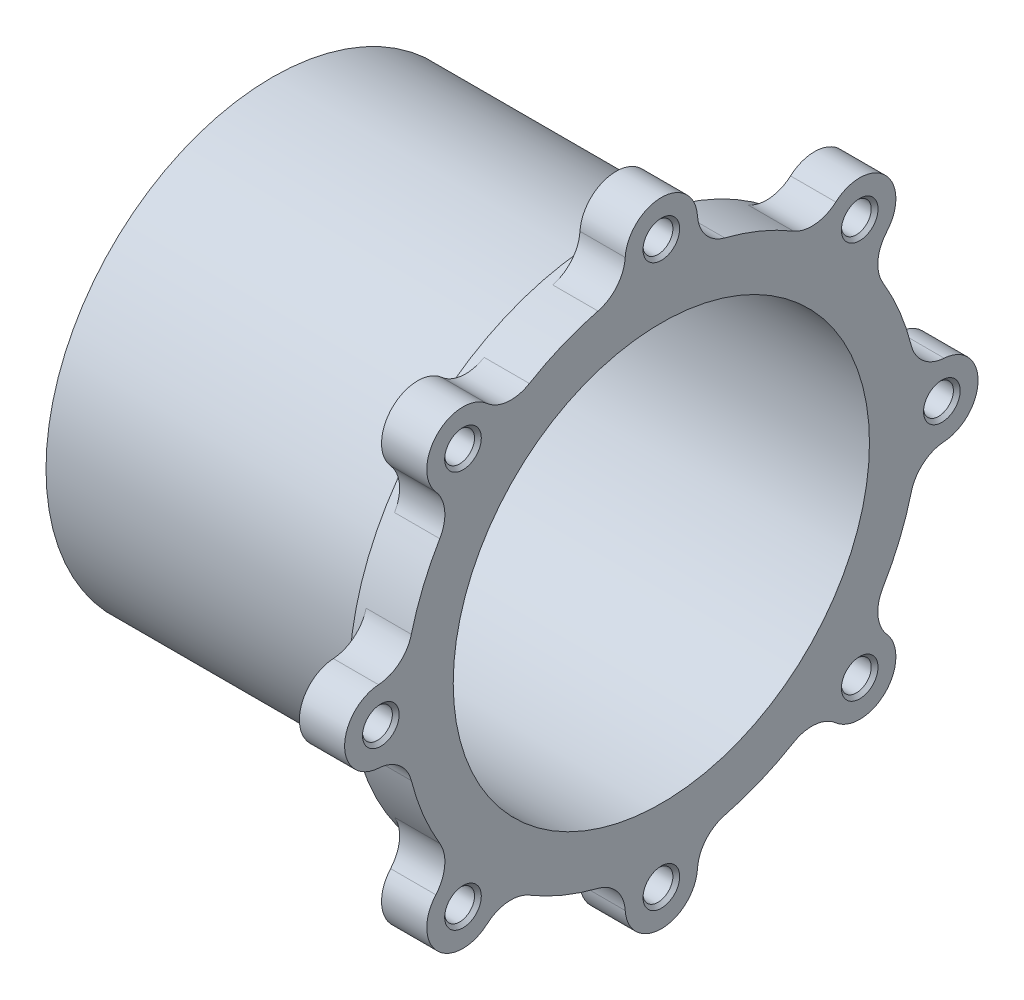
from build123d import *

# Parameters (mm, degrees)
SKETCH_2_R                   = 2.1
CUT_EXTRUDE_1_DEPTH          = 51.847812146
EXTRUDE_START                = 5
SKETCH_3_R                   = 35
SKETCH_3_R_2                 = 23
EXTRUDE_1_DEPTH              = 5
HOLE_WIZARD_M4_1_D           = 3.3
HOLE_WIZARD_M4_1_CSINK_D     = 4.05
HOLE_WIZARD_M4_1_CSINK_ANGLE = 90
CUT_EXTRUDE_3_DEPTH          = 420


with BuildPart() as part:
    # 草图1 → 旋转1 (revolve)
    with BuildSketch(Plane.XY, mode=Mode.PRIVATE) as revolve_1_sk:
        Polygon((0, 13.5), (0, 23), (28, 23), (28, 28.5), (27, 28.5), (27, 25), (-10, 25), (-10, 23), (-3, 23), (-3, 13.5), align=None)
    revolve(revolve_1_sk.sketch.rotate(Axis((-410.478449984, 0, 0), (1, 0, 0)), 90), axis=Axis((-410.478449984, 0, 0), (1, 0, 0)))

    # 草图2 → 切除-拉伸1 (cut, through all)
    with BuildSketch(Plane.ZY.offset(3)):
        with Locations((0, 17.5)):
            Circle(SKETCH_2_R)
        with Locations((12.374368671, 12.374368671)):
            Circle(SKETCH_2_R)
        with Locations((17.5, 0)):
            Circle(SKETCH_2_R)
        with Locations((12.374368671, -12.374368671)):
            Circle(SKETCH_2_R)
        with Locations((0, -17.5)):
            Circle(SKETCH_2_R)
        with Locations((-12.374368671, -12.374368671)):
            Circle(SKETCH_2_R)
        with Locations((-17.5, 0)):
            Circle(SKETCH_2_R)
        with Locations((-12.374368671, 12.374368671)):
            Circle(SKETCH_2_R)
    extrude(amount=-CUT_EXTRUDE_1_DEPTH, mode=Mode.SUBTRACT)

    # 草图3 → 凸台-拉伸1 (add)
    with BuildSketch(Plane(origin=(28, 0, 0), x_dir=(0, 0, -1), z_dir=(1, 0, 0)).offset(EXTRUDE_START)):
        Circle(SKETCH_3_R)
        with Locations(Location((0, 0, 0), (0, 0, 180))):
            Circle(SKETCH_3_R_2, mode=Mode.SUBTRACT)
    extrude(amount=-EXTRUDE_1_DEPTH)

    # M4 螺纹孔1 (through all)
    with Locations(Plane(origin=(33, 0, 0), x_dir=(0, 0, -1), z_dir=(1, 0, 0))):
        with Locations((-21.920310217, 21.920310217), (0, 31), (21.920310217, 21.920310217), (31, 0), (21.920310217, -21.920310217), (0, -31), (-21.920310217, -21.920310217), (-31, 0)):
            CounterSinkHole(HOLE_WIZARD_M4_1_D / 2, HOLE_WIZARD_M4_1_CSINK_D / 2, counter_sink_angle=HOLE_WIZARD_M4_1_CSINK_ANGLE)

    # 草图9 → 切除-拉伸3 (cut)
    with BuildSketch(Plane.ZY.offset(-28)):
        with BuildLine():
            ThreePointArc((0, 35), (2.737876502, 33.916167392), (3.99205309, 31.252016129))
            ThreePointArc((3.99205309, 31.252016129), (4.90631025, 28.949199149), (7.001446957, 27.626612903))
            ThreePointArc((7.001446957, 27.626612903), (10.906477822, 26.330566677), (14.584194703, 24.485735947))
            ThreePointArc((14.584194703, 24.485735947), (17.00088978, 23.939460276), (19.27570472, 24.921320341))
            ThreePointArc((19.27570472, 24.921320341), (22.046380914, 25.918322996), (24.748737342, 24.748737342))
            ThreePointArc((24.748737342, 24.748737342), (13.393920133, 32.335783638), (0, 35))
        make_face()
        with BuildLine():
            ThreePointArc((-3.99205309, 31.252016129), (-2.737876502, 33.916167392), (0, 35))
            ThreePointArc((0, 35), (-13.393920111, 32.335783647), (-24.748737308, 24.748737375))
            ThreePointArc((-24.748737308, 24.748737375), (-22.04638089, 25.918322996), (-19.27570472, 24.921320341))
            ThreePointArc((-19.27570472, 24.921320341), (-17.00088978, 23.939460276), (-14.584194703, 24.485735947))
            ThreePointArc((-14.584194703, 24.485735947), (-10.906477822, 26.330566677), (-7.001446957, 27.626612903))
            ThreePointArc((-7.001446957, 27.626612903), (-4.90631025, 28.949199149), (-3.99205309, 31.252016129))
        make_face()
        with BuildLine():
            ThreePointArc((35, 0), (32.335783638, 13.393920133), (24.748737342, 24.748737342))
            ThreePointArc((24.748737342, 24.748737342), (25.918322996, 22.046380914), (24.921320341, 19.27570472))
            ThreePointArc((24.921320341, 19.27570472), (23.939460276, 17.00088978), (24.485735947, 14.584194703))
            ThreePointArc((24.485735947, 14.584194703), (26.330566677, 10.906477822), (27.626612903, 7.001446957))
            ThreePointArc((27.626612903, 7.001446957), (28.949199149, 4.90631025), (31.252016129, 3.99205309))
            ThreePointArc((31.252016129, 3.99205309), (33.916167392, 2.737876502), (35, 0))
        make_face()
        with BuildLine():
            ThreePointArc((-24.921320341, 19.27570472), (-25.918322995, 22.046380937), (-24.748737308, 24.748737375))
            ThreePointArc((-24.748737308, 24.748737375), (-32.335783614, 13.39392019), (-35, 7.6e-08))
            ThreePointArc((-35, 7.6e-08), (-33.916167366, 2.73787653), (-31.252016129, 3.99205309))
            ThreePointArc((-31.252016129, 3.99205309), (-28.949199149, 4.90631025), (-27.626612903, 7.001446957))
            ThreePointArc((-27.626612903, 7.001446957), (-26.330566677, 10.906477822), (-24.485735947, 14.584194703))
            ThreePointArc((-24.485735947, 14.584194703), (-23.939460276, 17.00088978), (-24.921320341, 19.27570472))
        make_face()
        with BuildLine():
            ThreePointArc((24.748737305, -24.748737378), (32.335783628, -13.393920156), (35, 0))
            ThreePointArc((35, 0), (33.916167392, -2.737876502), (31.252016129, -3.99205309))
            ThreePointArc((31.252016129, -3.99205309), (28.949199149, -4.90631025), (27.626612903, -7.001446957))
            ThreePointArc((27.626612903, -7.001446957), (26.330566677, -10.906477822), (24.485735947, -14.584194703))
            ThreePointArc((24.485735947, -14.584194703), (23.939460276, -17.00088978), (24.921320341, -19.27570472))
            ThreePointArc((24.921320341, -19.27570472), (25.918322995, -22.046380939), (24.748737305, -24.748737378))
        make_face()
        with BuildLine():
            ThreePointArc((-31.252016129, -3.99205309), (-33.916167418, -2.737876475), (-35, 7.6e-08))
            ThreePointArc((-35, 7.6e-08), (-32.335783652, -13.393920098), (-24.748737342, -24.748737342))
            ThreePointArc((-24.748737342, -24.748737342), (-25.918322996, -22.046380914), (-24.921320341, -19.27570472))
            ThreePointArc((-24.921320341, -19.27570472), (-23.939460276, -17.00088978), (-24.485735947, -14.584194703))
            ThreePointArc((-24.485735947, -14.584194703), (-26.330566677, -10.906477822), (-27.626612903, -7.001446957))
            ThreePointArc((-27.626612903, -7.001446957), (-28.949199149, -4.90631025), (-31.252016129, -3.99205309))
        make_face()
        with BuildLine():
            ThreePointArc((0, -35), (13.393920109, -32.335783648), (24.748737305, -24.748737378))
            ThreePointArc((24.748737305, -24.748737378), (22.046380888, -25.918322996), (19.27570472, -24.921320341))
            ThreePointArc((19.27570472, -24.921320341), (17.00088978, -23.939460276), (14.584194703, -24.485735947))
            ThreePointArc((14.584194703, -24.485735947), (10.906477822, -26.330566677), (7.001446957, -27.626612903))
            ThreePointArc((7.001446957, -27.626612903), (4.90631025, -28.949199149), (3.99205309, -31.252016129))
            ThreePointArc((3.99205309, -31.252016129), (2.737876502, -33.916167392), (0, -35))
        make_face()
        with BuildLine():
            ThreePointArc((-19.27570472, -24.921320341), (-22.046380914, -25.918322996), (-24.748737342, -24.748737342))
            ThreePointArc((-24.748737342, -24.748737342), (-13.393920133, -32.335783638), (0, -35))
            ThreePointArc((0, -35), (-2.737876502, -33.916167392), (-3.99205309, -31.252016129))
            ThreePointArc((-3.99205309, -31.252016129), (-4.90631025, -28.949199149), (-7.001446957, -27.626612903))
            ThreePointArc((-7.001446957, -27.626612903), (-10.906477822, -26.330566677), (-14.584194703, -24.485735947))
            ThreePointArc((-14.584194703, -24.485735947), (-17.00088978, -23.939460276), (-19.27570472, -24.921320341))
        make_face()
    extrude(amount=-CUT_EXTRUDE_3_DEPTH, mode=Mode.SUBTRACT)


solid = part.part
